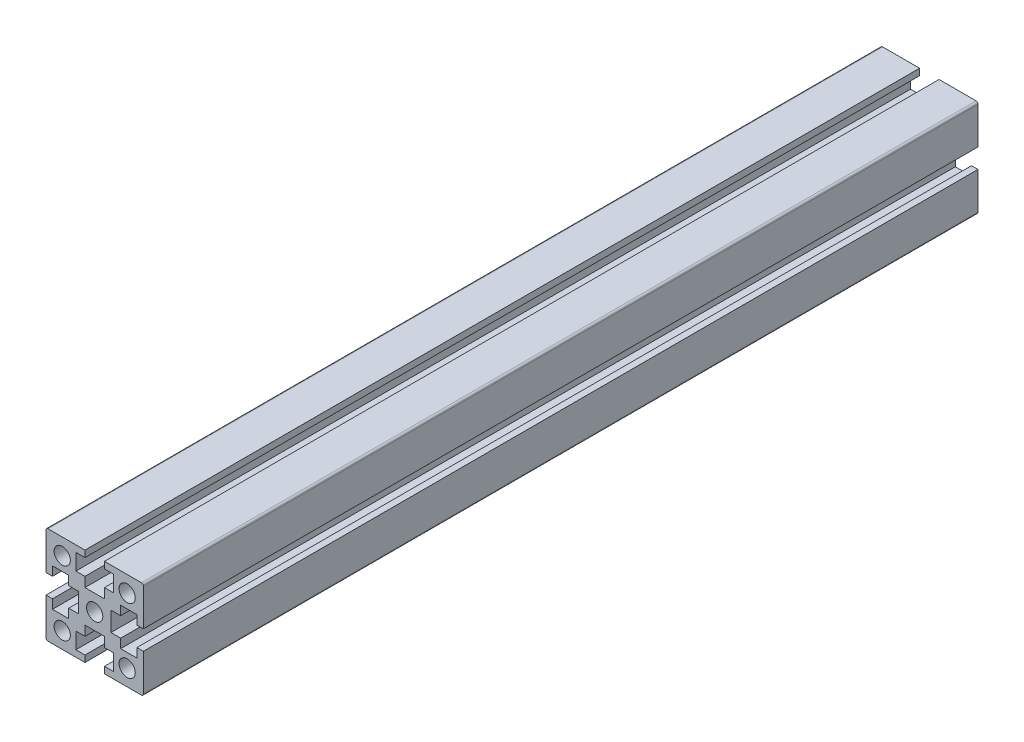
SolidWorks part; units mm, degrees
ref_plane "Front Plane" through (0, 0, 0) normal (0, 0, 1) x (1, 0, 0)
ref_plane "Top Plane" through (0, 0, 0) normal (0, 1, 0) x (1, 0, 0)
ref_plane "Right Plane" through (0, 0, 0) normal (1, 0, 0) x (0, 0, -1)
sketch "Sketch1" plane through (0, 0, 0) normal (0, 0, 1) x (1, 0, 0)
  line L1 (0, 0) -> (100, 0)
  line L2 (0, 0) -> (0, -6)
  line L3 (0, -6) -> (100, -6)
  line L4 (100, 0) -> (100, -6)
sketch "Sketch2" [suppressed] plane through (0, 0, 0) normal (0, 0, 1) x (1, 0, 0)
  line L0 (-23.6029, 0) -> (28.2626, 0) construction
  line L1 (-14, 15) -> (14, 15)
  line L2 (-15, 14) -> (-15, -14)
  line L3 (-14, -15) -> (14, -15)
  line L4 (15, 14) -> (15, -14)
  line L5 (-15, 15) -> (15, -15) construction
  line L6 (-15, -15) -> (15, 15) construction
  line L7 (0, 18.6426) -> (0, 15) construction
  line L8 (-6.45, 3.15) -> (-4.45, 3.15)
  line L9 (-15, 3.15) -> (-12.5, 3.15)
  line L10 (-15, 3.15) -> (-15, -3.15)
  line L11 (-15, -3.15) -> (-12.5, -3.15)
  line L12 (-4.45, 3.15) -> (-4.45, 0.5196)
  line L13 (-12.5, 5.15) -> (-6.45, 5.15)
  line L14 (-12.5, 5.15) -> (-12.5, 3.15)
  line L15 (-12.5, -5.15) -> (-12.5, -3.15)
  line L16 (-6.45, 5.15) -> (-6.45, 3.15)
  line L17 (-6.45, -5.15) -> (-6.45, -3.15)
  line L18 (-12.5, -5.15) -> (-6.45, -5.15)
  line L19 (-6.45, -3.15) -> (-4.45, -3.15)
  line L20 (3.15, 15) -> (3.15, 12.5)
  line L21 (5.15, 12.5) -> (3.15, 12.5)
  line L22 (5.15, 6.45) -> (3.15, 6.45)
  line L23 (5.15, 12.5) -> (5.15, 6.45)
  line L24 (3.15, 6.45) -> (3.15, 4.45)
  line L25 (-3.15, 15) -> (-3.15, 12.5)
  line L26 (-5.15, 12.5) -> (-3.15, 12.5)
  line L27 (-5.15, 12.5) -> (-5.15, 6.45)
  line L28 (-5.15, 6.45) -> (-3.15, 6.45)
  line L29 (-3.15, 6.45) -> (-3.15, 4.45)
  line L30 (-3.15, 4.45) -> (-0.5196, 4.45)
  line L31 (3.15, -4.45) -> (0.5196, -4.45)
  line L32 (-3.15, -6.45) -> (-3.15, -4.45)
  line L33 (-5.15, -6.45) -> (-3.15, -6.45)
  line L34 (-5.15, -12.5) -> (-5.15, -6.45)
  line L35 (-5.15, -12.5) -> (-3.15, -12.5)
  line L36 (-3.15, -15) -> (-3.15, -12.5)
  line L37 (3.15, -15) -> (3.15, -12.5)
  line L38 (5.15, -12.5) -> (3.15, -12.5)
  line L39 (5.15, -12.5) -> (5.15, -6.45)
  line L40 (5.15, -6.45) -> (3.15, -6.45)
  line L41 (3.15, -6.45) -> (3.15, -4.45)
  line L42 (6.45, -3.15) -> (4.45, -3.15)
  line L43 (6.45, -5.15) -> (6.45, -3.15)
  line L44 (12.5, -5.15) -> (6.45, -5.15)
  line L45 (12.5, -5.15) -> (12.5, -3.15)
  line L46 (15, -3.15) -> (12.5, -3.15)
  line L47 (15, 3.15) -> (12.5, 3.15)
  line L48 (12.5, 5.15) -> (12.5, 3.15)
  line L49 (12.5, 5.15) -> (6.45, 5.15)
  line L50 (6.45, 5.15) -> (6.45, 3.15)
  line L51 (6.45, 3.15) -> (4.45, 3.15)
  line L52 (4.45, -3.15) -> (4.45, -0.5196)
  line L53 (-0.5196, 4.45) -> (0, 4.15)
  line L54 (0.5196, 4.45) -> (0, 4.15)
  line L55 (0.5196, 4.45) -> (3.15, 4.45)
  line L56 (0, 4.15) -> (0, -17.8421) construction
  line L57 (4.45, 0.5196) -> (4.15, 0)
  line L58 (4.45, -0.5196) -> (4.15, 0)
  line L59 (-4.45, 0.5196) -> (-4.15, 0)
  line L60 (-4.45, -0.5196) -> (-4.15, 0)
  line L61 (-0.5196, -4.45) -> (0, -4.15)
  line L62 (0.5196, -4.45) -> (0, -4.15)
  line L63 (4.45, 0.5196) -> (4.45, 3.15)
  line L64 (-0.5196, -4.45) -> (-3.15, -4.45)
  line L65 (-4.45, -0.5196) -> (-4.45, -3.15)
  circle A0 centre (0, 0) radius 2.55
  circle A1 centre (-9.7, 9.7) radius 3.15
  circle A2 centre (9.7, -9.7) radius 3.15
  circle A3 centre (-9.7, -9.7) radius 3.15
  circle A4 centre (9.7, 9.7) radius 3.15
  arc A5 (-15, -14) -> (-14, -15) centre (-14, -14) ccw
  arc A6 (14, -15) -> (15, -14) centre (14, -14) ccw
  arc A7 (15, 14) -> (14, 15) centre (14, 14) ccw
  arc A8 (-14, 15) -> (-15, 14) centre (-14, 14) ccw
  point P0 (0, 0)
  dimension "D7" = 5.1
  dimension "D8" = 6.3
  dimension "D12" = 1
  dimension "D1" = 30
  dimension "D2" = 10.55
  dimension "D3" = 6.3
  dimension "D4" = 2
  dimension "D5" = 6.05
  dimension "D6" = 2.5
  dimension "D9" = 19.4
  dimension "D10" = 30
  dimension "D11" = 0.3
extrude "Boss-Extrude1" [suppressed] add sketch "Sketch2" along normal blind 100 contours L1 A8 L2 L9 L14 L13 L16 L8 L12 L59 L60 L65 L19 L17 L18 L15 L11 A5 L3 L36 L35 L34 L33 L32 L64 L61 L62 L31 L41 L40 L39 L38 L37 A6 L4 L46 L45 L44 L43 L42 L52 L58 L57 L63 L51 L50 L49 L48 L47
sketch "Sketch3" [suppressed] plane through (0, 0, 0) normal (0, 0, 1) x (1, 0, 0)
  line L0 (-35.5623, 0) -> (38.1151, 0) construction
  line L1 (-17, 20) -> (17, 20)
  line L2 (-20, 17) -> (-20, -17)
  line L3 (-17, -20) -> (17, -20)
  line L4 (20, 17) -> (20, -17)
  line L5 (-20, 20) -> (20, -20) construction
  line L6 (-20, -20) -> (20, 20) construction
  line L7 (0, 30.4074) -> (0, -29.6339) construction
  line L8 (-8.75, 4.25) -> (-6, 4.25)
  line L9 (-20, 4.25) -> (-16.5, 4.25)
  line L10 (-20, 4.25) -> (-20, -4.25)
  line L11 (-20, -4.25) -> (-16.5, -4.25)
  line L12 (-6, 4.25) -> (-6, -4.25)
  line L13 (-8.75, -4.25) -> (-8.75, -7)
  line L14 (-16.5, 4.25) -> (-16.5, 7)
  line L15 (-16.5, 7) -> (-8.75, 7)
  line L16 (-8.75, 4.25) -> (-8.75, 7)
  line L17 (-16.5, -4.25) -> (-16.5, -7)
  line L18 (-16.5, -7) -> (-8.75, -7)
  line L19 (-8.75, -4.25) -> (-6, -4.25)
  line L20 (20, -4.25) -> (16.5, -4.25)
  line L21 (16.5, -4.25) -> (16.5, -7)
  line L22 (16.5, -7) -> (8.75, -7)
  line L23 (8.75, -4.25) -> (8.75, -7)
  line L24 (8.75, -4.25) -> (6, -4.25)
  line L25 (20, 4.25) -> (16.5, 4.25)
  line L26 (16.5, 4.25) -> (16.5, 7)
  line L27 (16.5, 7) -> (8.75, 7)
  line L28 (8.75, 4.25) -> (8.75, 7)
  line L29 (8.75, 4.25) -> (6, 4.25)
  line L30 (6, 4.25) -> (6, -4.25)
  line L31 (4.25, -8.75) -> (4.25, -6)
  line L32 (4.25, -8.75) -> (7, -8.75)
  line L33 (7, -16.5) -> (7, -8.75)
  line L34 (4.25, -16.5) -> (7, -16.5)
  line L35 (4.25, -20) -> (4.25, -16.5)
  line L36 (-4.25, -20) -> (-4.25, -16.5)
  line L37 (-4.25, -6) -> (4.25, -6)
  line L38 (-4.25, 8.75) -> (-4.25, 6)
  line L39 (-4.25, 8.75) -> (-7, 8.75)
  line L40 (-7, 16.5) -> (-7, 8.75)
  line L41 (-4.25, 16.5) -> (-7, 16.5)
  line L42 (-4.25, 20) -> (-4.25, 16.5)
  line L43 (-4.25, 6) -> (4.25, 6)
  line L44 (-4.25, -16.5) -> (-7, -16.5)
  line L45 (-4.25, -8.75) -> (-4.25, -6)
  line L46 (-4.25, -8.75) -> (-7, -8.75)
  line L47 (-7, -16.5) -> (-7, -8.75)
  line L48 (4.25, 20) -> (4.25, 16.5)
  line L49 (7, 16.5) -> (7, 8.75)
  line L50 (4.25, 16.5) -> (7, 16.5)
  line L51 (4.25, 8.75) -> (4.25, 6)
  line L52 (4.25, 8.75) -> (7, 8.75)
  circle A0 centre (0, 0) radius 4.4
  circle A1 centre (-13.5, 13.5) radius 5
  circle A2 centre (-13.5, -13.5) radius 5
  circle A3 centre (13.5, -13.5) radius 5
  circle A4 centre (13.5, 13.5) radius 5
  arc A5 (-20, -17) -> (-17, -20) centre (-17, -17) ccw
  arc A6 (17, -20) -> (20, -17) centre (17, -17) ccw
  arc A7 (20, 17) -> (17, 20) centre (17, 17) ccw
  arc A8 (-17, 20) -> (-20, 17) centre (-17, 17) ccw
  point P0 (0, 0)
  dimension "D2" = 8.8
  dimension "D3" = 10
  dimension "D10" = 3
  dimension "D1" = 40
  dimension "D4" = 8.5
  dimension "D5" = 14
  dimension "D6" = 14
  dimension "D7" = 2.75
  dimension "D8" = 3.5
  dimension "D9" = 6.5
extrude "Boss-Extrude2" [suppressed] add sketch "Sketch3" along normal blind 100 contours L1 A8 L2 L9 L14 L15 L16 L8 L12 L19 L13 L18 L17 L11 A5 L3 L36 L44 L47 L46 L45 L37 L31 L32 L33 L34 L35 A6 L4 L20 L21 L22 L23 L24 L30 L29 L28 L27 L26 L25 A7 L48 L50 L49 L52 L51 L43
sketch "Sketch4" plane through (0, 0, 0) normal (0, 0, 1) x (1, 0, 0)
  line L0 (-10.7398, 0) -> (11.0932, 0) construction
  line L1 (-7.2, 7.5) -> (7.2, 7.5)
  line L2 (-7.5, 7.2) -> (-7.5, -7.2)
  line L3 (-7.2, -7.5) -> (7.2, -7.5)
  line L4 (7.5, 7.2) -> (7.5, -7.2)
  line L5 (-7.5, 7.5) -> (7.5, -7.5) construction
  line L6 (-7.5, -7.5) -> (7.5, 7.5) construction
  line L7 (0, 10.0417) -> (0, -9.5776) construction
  line L8 (-1.5, 4) -> (-1.5, 2.5)
  line L9 (-1.5, 7.5) -> (1.5, 7.5)
  line L10 (-1.5, 7.5) -> (-1.5, 6.5)
  line L11 (-1.5, 2.5) -> (1.5, 2.5)
  line L12 (1.5, 7.5) -> (1.5, 6.5)
  line L13 (-1.5, 6.5) -> (-2.9, 6.5)
  line L14 (1.5, 4) -> (1.5, 2.5)
  line L15 (-1.5, 4) -> (-2.9, 4)
  line L16 (-2.9, 6.5) -> (-2.9, 4)
  line L17 (1.5, 4) -> (2.9, 4)
  line L18 (1.5, 7.5) -> (1.5, 6.5)
  line L19 (1.5, 6.5) -> (2.9, 6.5)
  line L20 (2.9, 6.5) -> (2.9, 4)
  line L21 (1.5, 4) -> (1.5, 2.5)
  line L22 (4, -1.5) -> (4, -2.9)
  line L23 (4, -1.5) -> (2.5, -1.5)
  line L24 (2.5, -1.5) -> (2.5, 1.5)
  line L25 (4, 1.5) -> (2.5, 1.5)
  line L26 (4, 1.5) -> (4, 2.9)
  line L27 (6.5, 2.9) -> (4, 2.9)
  line L28 (6.5, 1.5) -> (6.5, 2.9)
  line L29 (7.5, 1.5) -> (6.5, 1.5)
  line L30 (7.5, -1.5) -> (6.5, -1.5)
  line L31 (6.5, -1.5) -> (6.5, -2.9)
  line L32 (6.5, -2.9) -> (4, -2.9)
  line L33 (1.5, -7.5) -> (1.5, -6.5)
  line L34 (1.5, -6.5) -> (2.9, -6.5)
  line L35 (2.9, -6.5) -> (2.9, -4)
  line L36 (1.5, -4) -> (2.9, -4)
  line L37 (1.5, -4) -> (1.5, -2.5)
  line L38 (1.5, -2.5) -> (-1.5, -2.5)
  line L39 (-1.5, -4) -> (-1.5, -2.5)
  line L40 (-1.5, -7.5) -> (-1.5, -6.5)
  line L41 (-1.5, -6.5) -> (-2.9, -6.5)
  line L42 (-2.9, -6.5) -> (-2.9, -4)
  line L43 (-1.5, -4) -> (-2.9, -4)
  line L44 (-4, 1.5) -> (-4, 2.9)
  line L45 (-4, 1.5) -> (-2.5, 1.5)
  line L46 (-2.5, 1.5) -> (-2.5, -1.5)
  line L47 (-4, -1.5) -> (-2.5, -1.5)
  line L48 (-4, -1.5) -> (-4, -2.9)
  line L49 (-6.5, -2.9) -> (-4, -2.9)
  line L50 (-6.5, -1.5) -> (-6.5, -2.9)
  line L51 (-7.5, -1.5) -> (-6.5, -1.5)
  line L52 (-7.5, 1.5) -> (-6.5, 1.5)
  line L53 (-6.5, 1.5) -> (-6.5, 2.9)
  line L54 (-6.5, 2.9) -> (-4, 2.9)
  circle A0 centre (-5, 5) radius 1.25
  circle A1 centre (0, 0) radius 1.25
  circle A2 centre (5, 5) radius 1.25
  circle A3 centre (5, -5) radius 1.25
  circle A4 centre (-5, -5) radius 1.25
  arc A5 (-7.5, -7.2) -> (-7.2, -7.5) centre (-7.2, -7.2) ccw
  arc A6 (7.2, -7.5) -> (7.5, -7.2) centre (7.2, -7.2) ccw
  arc A7 (7.5, 7.2) -> (7.2, 7.5) centre (7.2, 7.2) ccw
  arc A8 (-7.2, 7.5) -> (-7.5, 7.2) centre (-7.2, 7.2) ccw
  point P0 (0, 0)
  dimension "D2" = 2.5
  dimension "D3" = 2.5
  dimension "D10" = 0.3
  dimension "D1" = 15
  dimension "D4" = 10
  dimension "D5" = 3
  dimension "D6" = 5
  dimension "D7" = 1
  dimension "D8" = 2.5
  dimension "D9" = 1.4
extrude "Boss-Extrude3" add sketch "Sketch4" along normal blind 100 contours L1 A8 L2 L52 L53 L54 L44 L45 L46 L47 L48 L49 L50 L51 A5 L3 L40 L41 L42 L43 L39 L38 L37 L36 L35 L34 L33 A6 L4 L30 L31 L32 L22 L23 L24 L25 L26 L27 L28 L29 A7 L12 L19 L20 L17 L14 L11
scale "Scale 1" bodies to scale 108 scale about origin uniform scaling yes scale factor 0.7
sketch "Sketch5" plane through (0, 0, 70) normal (0, 0, 1) x (1, 0, 0)
  line L52 (-1.05, 5.25) -> (-5.04, 5.25)
  line L53 (-5.25, 5.04) -> (-5.25, 1.05)
  line L54 (-5.25, 1.05) -> (-4.55, 1.05)
  line L55 (-4.55, 1.05) -> (-4.55, 2.03)
  line L56 (-4.55, 2.03) -> (-2.8, 2.03)
  line L57 (-2.8, 2.03) -> (-2.8, 1.05)
  line L58 (-2.8, 1.05) -> (-1.75, 1.05)
  line L59 (-1.75, 1.05) -> (-1.75, -1.05)
  line L60 (-1.75, -1.05) -> (-2.8, -1.05)
  line L61 (-2.8, -1.05) -> (-2.8, -2.03)
  line L62 (-2.8, -2.03) -> (-4.55, -2.03)
  line L63 (-4.55, -2.03) -> (-4.55, -1.05)
  line L64 (-4.55, -1.05) -> (-5.25, -1.05)
  line L65 (-5.25, -1.05) -> (-5.25, -5.04)
  line L66 (-5.04, -5.25) -> (-1.05, -5.25)
  line L67 (-1.05, -5.25) -> (-1.05, -4.55)
  line L68 (-1.05, -4.55) -> (-2.03, -4.55)
  line L69 (-2.03, -4.55) -> (-2.03, -2.8)
  line L70 (-2.03, -2.8) -> (-1.05, -2.8)
  line L71 (-1.05, -2.8) -> (-1.05, -1.75)
  line L72 (-1.05, -1.75) -> (1.05, -1.75)
  line L73 (1.05, -1.75) -> (1.05, -2.8)
  line L74 (1.05, -2.8) -> (2.03, -2.8)
  line L75 (2.03, -2.8) -> (2.03, -4.55)
  line L76 (2.03, -4.55) -> (1.05, -4.55)
  line L77 (1.05, -4.55) -> (1.05, -5.25)
  line L78 (1.05, -5.25) -> (5.04, -5.25)
  line L79 (5.25, -5.04) -> (5.25, -1.05)
  line L80 (5.25, -1.05) -> (4.55, -1.05)
  line L81 (4.55, -1.05) -> (4.55, -2.03)
  line L82 (4.55, -2.03) -> (2.8, -2.03)
  line L83 (2.8, -2.03) -> (2.8, -1.05)
  line L84 (2.8, -1.05) -> (1.75, -1.05)
  line L85 (1.75, -1.05) -> (1.75, 1.05)
  line L86 (1.75, 1.05) -> (2.8, 1.05)
  line L87 (2.8, 1.05) -> (2.8, 2.03)
  line L88 (2.8, 2.03) -> (4.55, 2.03)
  line L89 (4.55, 2.03) -> (4.55, 1.05)
  line L90 (4.55, 1.05) -> (5.25, 1.05)
  line L91 (5.25, 1.05) -> (5.25, 5.04)
  line L92 (5.04, 5.25) -> (1.05, 5.25)
  line L93 (1.05, 5.25) -> (1.05, 4.55)
  line L94 (1.05, 4.55) -> (2.03, 4.55)
  line L95 (2.03, 4.55) -> (2.03, 2.8)
  line L96 (2.03, 2.8) -> (1.05, 2.8)
  line L97 (1.05, 2.8) -> (1.05, 1.75)
  line L98 (1.05, 1.75) -> (-1.05, 1.75)
  line L99 (-1.05, 1.75) -> (-1.05, 2.8)
  line L100 (-1.05, 2.8) -> (-2.03, 2.8)
  line L101 (-2.03, 2.8) -> (-2.03, 4.55)
  line L102 (-2.03, 4.55) -> (-1.05, 4.55)
  line L103 (-1.05, 4.55) -> (-1.05, 5.25)
  line L104 (-1.05, 5.25) -> (-5.04, 5.25)
  line L105 (-5.25, 5.04) -> (-5.25, 1.05)
  line L106 (-5.25, 1.05) -> (-4.55, 1.05)
  line L107 (-4.55, 1.05) -> (-4.55, 2.03)
  line L108 (-4.55, 2.03) -> (-2.8, 2.03)
  line L109 (-2.8, 2.03) -> (-2.8, 1.05)
  line L110 (-2.8, 1.05) -> (-1.75, 1.05)
  line L111 (-1.75, 1.05) -> (-1.75, -1.05)
  line L112 (-1.75, -1.05) -> (-2.8, -1.05)
  line L113 (-2.8, -1.05) -> (-2.8, -2.03)
  line L114 (-2.8, -2.03) -> (-4.55, -2.03)
  line L115 (-4.55, -2.03) -> (-4.55, -1.05)
  line L116 (-4.55, -1.05) -> (-5.25, -1.05)
  line L117 (-5.25, -1.05) -> (-5.25, -5.04)
  line L118 (-5.04, -5.25) -> (-1.05, -5.25)
  line L119 (-1.05, -5.25) -> (-1.05, -4.55)
  line L120 (-1.05, -4.55) -> (-2.03, -4.55)
  line L121 (-2.03, -4.55) -> (-2.03, -2.8)
  line L122 (-2.03, -2.8) -> (-1.05, -2.8)
  line L123 (-1.05, -2.8) -> (-1.05, -1.75)
  line L124 (-1.05, -1.75) -> (1.05, -1.75)
  line L125 (1.05, -1.75) -> (1.05, -2.8)
  line L126 (1.05, -2.8) -> (2.03, -2.8)
  line L127 (2.03, -2.8) -> (2.03, -4.55)
  line L128 (2.03, -4.55) -> (1.05, -4.55)
  line L129 (1.05, -4.55) -> (1.05, -5.25)
  line L130 (1.05, -5.25) -> (5.04, -5.25)
  line L131 (5.25, -5.04) -> (5.25, -1.05)
  line L132 (5.25, -1.05) -> (4.55, -1.05)
  line L133 (4.55, -1.05) -> (4.55, -2.03)
  line L134 (4.55, -2.03) -> (2.8, -2.03)
  line L135 (2.8, -2.03) -> (2.8, -1.05)
  line L136 (2.8, -1.05) -> (1.75, -1.05)
  line L137 (1.75, -1.05) -> (1.75, 1.05)
  line L138 (1.75, 1.05) -> (2.8, 1.05)
  line L139 (2.8, 1.05) -> (2.8, 2.03)
  line L140 (2.8, 2.03) -> (4.55, 2.03)
  line L141 (4.55, 2.03) -> (4.55, 1.05)
  line L142 (4.55, 1.05) -> (5.25, 1.05)
  line L143 (5.25, 1.05) -> (5.25, 5.04)
  line L144 (5.04, 5.25) -> (1.05, 5.25)
  line L145 (1.05, 5.25) -> (1.05, 4.55)
  line L146 (1.05, 4.55) -> (2.03, 4.55)
  line L147 (2.03, 4.55) -> (2.03, 2.8)
  line L148 (2.03, 2.8) -> (1.05, 2.8)
  line L149 (1.05, 2.8) -> (1.05, 1.75)
  line L150 (1.05, 1.75) -> (-1.05, 1.75)
  line L151 (-1.05, 1.75) -> (-1.05, 2.8)
  line L152 (-1.05, 2.8) -> (-2.03, 2.8)
  line L153 (-2.03, 2.8) -> (-2.03, 4.55)
  line L154 (-2.03, 4.55) -> (-1.05, 4.55)
  line L155 (-1.05, 4.55) -> (-1.05, 5.25)
  circle A0 centre (3.5, -3.5) radius 0.875 construction
  circle A1 centre (-3.5, -3.5) radius 0.875 construction
  circle A2 centre (-3.5, 3.5) radius 0.875 construction
  circle A3 centre (3.5, 3.5) radius 0.875 construction
  arc A4 (-5.04, 5.25) -> (-5.25, 5.04) centre (-5.04, 5.04) ccw
  arc A5 (-5.25, -5.04) -> (-5.04, -5.25) centre (-5.04, -5.04) ccw
  arc A6 (5.04, -5.25) -> (5.25, -5.04) centre (5.04, -5.04) ccw
  arc A7 (5.25, 5.04) -> (5.04, 5.25) centre (5.04, 5.04) ccw
  arc A8 (-5.04, 5.25) -> (-5.25, 5.04) centre (-5.04, 5.04) ccw
  arc A9 (-5.25, -5.04) -> (-5.04, -5.25) centre (-5.04, -5.04) ccw
  arc A10 (5.04, -5.25) -> (5.25, -5.04) centre (5.04, -5.04) ccw
  arc A11 (5.25, 5.04) -> (5.04, 5.25) centre (5.04, 5.04) ccw
  circle A12 centre (0, 0) radius 0.875 construction
  circle A13 centre (3.5, -3.5) radius 0.875
  circle A14 centre (-3.5, -3.5) radius 0.875
  circle A15 centre (-3.5, 3.5) radius 0.875
  circle A16 centre (3.5, 3.5) radius 0.875
  circle A17 centre (0, 0) radius 0.875
  dimension "D1" = 0
extrude "Boss-Extrude4" add sketch "Sketch5" along normal blind 20
equation "\"D1@Boss-Extrude1\" = \"L@Sketch1\""
equation "\"D1@Boss-Extrude2\" = \"L@Sketch1\""
equation "\"D1@Boss-Extrude3\" = \"L@Sketch1\""
